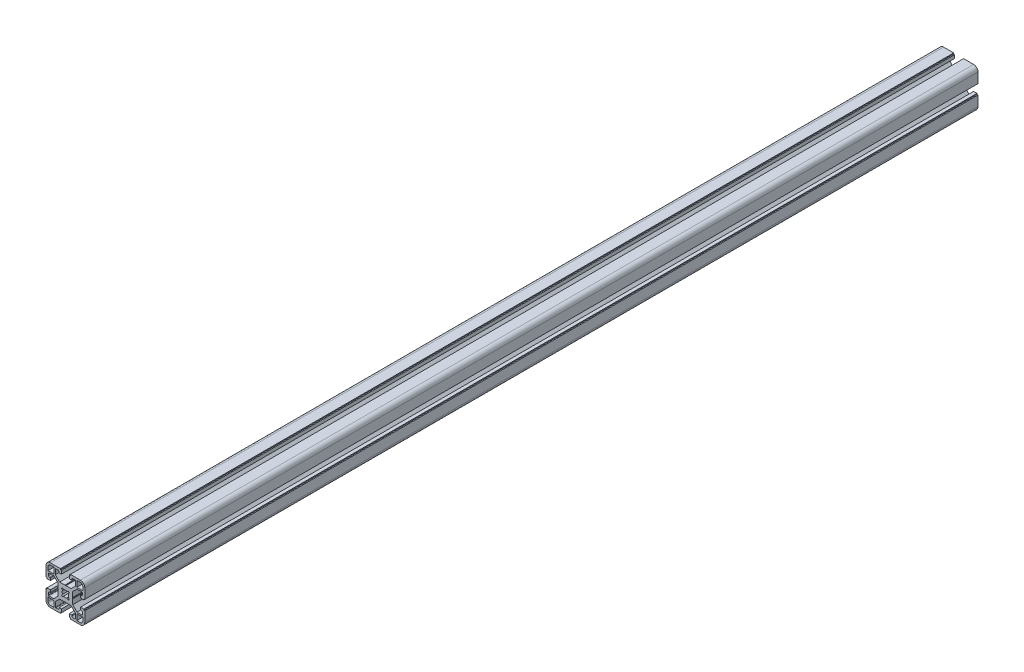
SolidWorks part; units mm, degrees
material "6061 GB/T6892-2006"
ref_plane "前视" through (0, 0, 0) normal (0, 0, 1) x (1, 0, 0)
ref_plane "上视" through (0, 0, 0) normal (0, 1, 0) x (1, 0, 0)
ref_plane "右视" through (0, 0, 0) normal (1, 0, 0) x (0, 0, -1)
sketch "草图1" plane through (0, 0, 0) normal (0, 0, 1) x (1, 0, 0)
  line L0 (-18.9995, -4.1003) -> (-18.9995, -5.1003)
  line L1 (-18.9995, -5.1003) -> (-19.9995, -5.1003)
  line L2 (-19.9995, -5.1003) -> (-19.9995, -15.5003)
  line L3 (-15.4995, -20.0003) -> (-5.0995, -20.0003)
  line L4 (-5.0995, -20.0003) -> (-5.0995, -19.0003)
  line L5 (-5.0995, -19.0003) -> (-4.0995, -19.0003)
  line L6 (-4.0995, -19.0003) -> (-4.0995, -15.5003)
  line L7 (-4.0995, -15.5003) -> (-6.5995, -15.5003)
  line L8 (-6.5995, -15.5003) -> (-6.5995, -16.5003)
  line L9 (-7.5995, -17.5003) -> (-9.7995, -17.5003)
  line L10 (-10.2995, -17.0003) -> (-10.2995, -11.9973)
  line L11 (-10.2995, -11.9973) -> (-5.9025, -7.6003)
  line L12 (-5.9025, -7.6003) -> (-0.5195, -7.6003)
  line L13 (-0.5195, -7.6003) -> (0.0005, -7.3003)
  line L14 (0.0005, -7.3003) -> (0.5195, -7.6003)
  line L15 (0.5195, -7.6003) -> (5.9035, -7.6003)
  line L16 (5.9035, -7.6003) -> (10.3005, -11.9973)
  line L17 (10.3005, -11.9973) -> (10.3005, -17.0003)
  line L18 (9.8005, -17.5003) -> (7.6005, -17.5003)
  line L19 (6.6005, -16.5003) -> (6.6005, -15.5003)
  line L20 (6.6005, -15.5003) -> (4.1005, -15.5003)
  line L21 (4.1005, -15.5003) -> (4.1005, -19.0003)
  line L22 (4.1005, -19.0003) -> (5.1005, -19.0003)
  line L23 (5.1005, -19.0003) -> (5.1005, -20.0003)
  line L24 (5.1005, -20.0003) -> (15.5005, -20.0003)
  line L25 (20.0005, -15.5003) -> (20.0005, -5.1003)
  line L26 (20.0005, -5.1003) -> (19.0005, -5.1003)
  line L27 (19.0005, -5.1003) -> (19.0005, -4.1003)
  line L28 (19.0005, -4.1003) -> (15.5005, -4.1003)
  line L29 (15.5005, -4.1003) -> (15.5005, -6.6003)
  line L30 (15.5005, -6.6003) -> (16.5005, -6.6003)
  line L31 (17.5005, -7.6003) -> (17.5005, -9.8003)
  line L32 (17.0005, -10.3003) -> (11.9975, -10.3003)
  line L33 (11.9975, -10.3003) -> (7.6005, -5.9033)
  line L34 (7.6005, -5.9033) -> (7.6005, -0.5203)
  line L35 (7.6005, -0.5203) -> (7.3005, -0.0003)
  line L36 (7.3005, -0.0003) -> (7.6005, 0.5197)
  line L37 (7.6005, 0.5197) -> (7.6005, 5.9027)
  line L38 (7.6005, 5.9027) -> (11.9975, 10.2997)
  line L39 (11.9975, 10.2997) -> (17.0005, 10.2997)
  line L40 (17.5005, 9.7997) -> (17.5005, 7.5997)
  line L41 (16.5005, 6.5997) -> (15.5005, 6.5997)
  line L42 (15.5005, 6.5997) -> (15.5005, 4.0997)
  line L43 (15.5005, 4.0997) -> (19.0005, 4.0997)
  line L44 (19.0005, 4.0997) -> (19.0005, 5.0997)
  line L45 (19.0005, 5.0997) -> (20.0005, 5.0997)
  line L46 (20.0005, 5.0997) -> (20.0005, 15.4997)
  line L47 (15.5005, 19.9997) -> (5.1005, 19.9997)
  line L48 (5.1005, 19.9997) -> (5.1005, 18.9997)
  line L49 (5.1005, 18.9997) -> (4.1005, 18.9997)
  line L50 (4.1005, 18.9997) -> (4.1005, 15.4997)
  line L51 (4.1005, 15.4997) -> (6.6005, 15.4997)
  line L52 (7.6005, 17.4997) -> (9.8005, 17.4997)
  line L53 (10.3005, 16.9997) -> (10.3005, 11.9967)
  line L54 (10.3005, 11.9967) -> (5.9035, 7.5997)
  line L55 (5.9035, 7.5997) -> (0.5195, 7.5997)
  line L56 (0.5195, 7.5997) -> (0.0005, 7.2997)
  line L57 (0.0005, 7.2997) -> (-0.5195, 7.5997)
  line L58 (-0.5195, 7.5997) -> (-5.9025, 7.5997)
  line L59 (-5.9025, 7.5997) -> (-10.2995, 11.9967)
  line L60 (-10.2995, 11.9967) -> (-10.2995, 16.9997)
  line L61 (-9.7995, 17.4997) -> (-7.5995, 17.4997)
  line L62 (-6.5995, 16.4997) -> (-6.5995, 15.4997)
  line L63 (-6.5995, 15.4997) -> (-4.0995, 15.4997)
  line L64 (-4.0995, 15.4997) -> (-4.0995, 18.9997)
  line L65 (-4.0995, 18.9997) -> (-5.0995, 18.9997)
  line L66 (-5.0995, 18.9997) -> (-5.0995, 19.9997)
  line L67 (-5.0995, 19.9997) -> (-15.4995, 19.9997)
  line L68 (-19.9995, 15.4997) -> (-19.9995, 5.0997)
  line L69 (-19.9995, 5.0997) -> (-18.9995, 5.0997)
  line L70 (-18.9995, 5.0997) -> (-18.9995, 4.0997)
  line L71 (-18.9995, 4.0997) -> (-15.4995, 4.0997)
  line L72 (-15.4995, 4.0997) -> (-15.4995, 6.5997)
  line L73 (-15.4995, 6.5997) -> (-16.4995, 6.5997)
  line L74 (-17.4995, 7.5997) -> (-17.4995, 9.7997)
  line L75 (-16.9995, 10.2997) -> (-11.9965, 10.2997)
  line L76 (-11.9965, 10.2997) -> (-7.5995, 5.9027)
  line L77 (-7.5995, 5.9027) -> (-7.5995, 0.5197)
  line L78 (-7.5995, 0.5197) -> (-7.2995, -0.0003)
  line L79 (-7.2995, -0.0003) -> (-7.5995, -0.5203)
  line L80 (-7.5995, -0.5203) -> (-7.5995, -5.9033)
  line L81 (-7.5995, -5.9033) -> (-11.9965, -10.3003)
  line L82 (-11.9965, -10.3003) -> (-16.9995, -10.3003)
  line L83 (-17.4995, -9.8003) -> (-17.4995, -7.6003)
  line L84 (-16.4995, -6.6003) -> (-15.4995, -6.6003)
  line L85 (-15.4995, -6.6003) -> (-15.4995, -4.1003)
  line L86 (-15.4995, -4.1003) -> (-18.9995, -4.1003)
  line L87 (15.5005, -18.0003) -> (11.8005, -18.0003)
  line L88 (11.8005, -18.0003) -> (11.8005, -11.8003)
  line L89 (11.8005, -11.8003) -> (18.0005, -11.8003)
  line L90 (18.0005, -11.8003) -> (18.0005, -15.5003)
  line L91 (18.0005, 11.7997) -> (11.8005, 11.7997)
  line L92 (11.8005, 11.7997) -> (11.8005, 17.9997)
  line L93 (11.8005, 17.9997) -> (15.5005, 17.9997)
  line L94 (18.0005, 15.4997) -> (18.0005, 11.7997)
  line L95 (-1.8145, -2.8753) -> (-3.0044, -4.0665)
  line L96 (-3.0044, -4.0665) -> (-4.0656, -3.0052)
  line L97 (-4.0656, -3.0052) -> (-2.8745, -1.8153)
  line L98 (-2.8745, 1.8147) -> (-4.0644, 3.0058)
  line L99 (-4.0644, 3.0058) -> (-3.0044, 4.0658)
  line L100 (-3.0044, 4.0658) -> (-1.8145, 2.8747)
  line L101 (1.8145, 2.8747) -> (3.0055, 4.0657)
  line L102 (3.0055, 4.0657) -> (4.0666, 3.0045)
  line L103 (4.0666, 3.0045) -> (2.8755, 1.8147)
  line L104 (2.8755, -1.8153) -> (4.0666, -3.0052)
  line L105 (4.0666, -3.0052) -> (3.0055, -4.0663)
  line L106 (3.0055, -4.0663) -> (1.8145, -2.8753)
  line L107 (-17.9995, -15.5003) -> (-17.9995, -11.8003)
  line L108 (-17.9995, -11.8003) -> (-11.7995, -11.8003)
  line L109 (-11.7995, -11.8003) -> (-11.7995, -18.0003)
  line L110 (-11.7995, -18.0003) -> (-15.4995, -18.0003)
  line L111 (-11.7995, 17.9997) -> (-11.7995, 11.7997)
  line L112 (-11.7995, 11.7997) -> (-17.9995, 11.7997)
  line L113 (-17.9995, 11.7997) -> (-17.9995, 15.4997)
  line L114 (-15.4995, 17.9997) -> (-11.7995, 17.9997)
  arc A0 (-19.9995, -15.5003) -> (-15.4995, -20.0003) centre (-15.4995, -15.5003) ccw
  arc A1 (-6.5995, -16.5003) -> (-7.5995, -17.5003) centre (-7.5995, -16.5003) cw
  arc A2 (-9.7995, -17.5003) -> (-10.2995, -17.0003) centre (-9.7995, -17.0003) cw
  arc A3 (10.3005, -17.0003) -> (9.8005, -17.5003) centre (9.8005, -17.0003) cw
  arc A4 (7.6005, -17.5003) -> (6.6005, -16.5003) centre (7.6005, -16.5003) cw
  arc A5 (15.5005, -20.0003) -> (20.0005, -15.5003) centre (15.5005, -15.5003) ccw
  arc A6 (16.5005, -6.6003) -> (17.5005, -7.6003) centre (16.5005, -7.6003) cw
  arc A7 (17.5005, -9.8003) -> (17.0005, -10.3003) centre (17.0005, -9.8003) cw
  arc A8 (17.0005, 10.2997) -> (17.5005, 9.7997) centre (17.0005, 9.7997) cw
  arc A9 (17.5005, 7.5997) -> (16.5005, 6.5997) centre (16.5005, 7.5997) cw
  arc A10 (20.0005, 15.4997) -> (15.5005, 19.9997) centre (15.5005, 15.4997) ccw
  arc A11 (6.6005, 15.4997) -> (6.6005, 16.4997) centre (7.1003, 15.9997) cw
  arc A12 (6.6005, 16.4997) -> (7.6005, 17.4997) centre (7.6005, 16.4997) cw
  arc A13 (9.8005, 17.4997) -> (10.3005, 16.9997) centre (9.8005, 16.9997) cw
  arc A14 (-10.2995, 16.9997) -> (-9.7995, 17.4997) centre (-9.7995, 16.9997) cw
  arc A15 (-7.5995, 17.4997) -> (-6.5995, 16.4997) centre (-7.5995, 16.4997) cw
  arc A16 (-15.4995, 19.9997) -> (-19.9995, 15.4997) centre (-15.4995, 15.4997) ccw
  arc A17 (-16.4995, 6.5997) -> (-17.4995, 7.5997) centre (-16.4995, 7.5997) cw
  arc A18 (-17.4995, 9.7997) -> (-16.9995, 10.2997) centre (-16.9995, 9.7997) cw
  arc A19 (-16.9995, -10.3003) -> (-17.4995, -9.8003) centre (-16.9995, -9.8003) cw
  arc A20 (-17.4995, -7.6003) -> (-16.4995, -6.6003) centre (-16.4995, -7.6003) cw
  arc A21 (18.0005, -15.5003) -> (15.5005, -18.0003) centre (15.5005, -15.5003) cw
  arc A22 (15.5005, 17.9997) -> (18.0005, 15.4997) centre (15.5005, 15.4997) cw
  arc A23 (-2.8745, -1.8153) -> (-2.8745, 1.8147) centre (0.0005, -0.0003) cw
  arc A24 (-1.8145, 2.8747) -> (1.8145, 2.8747) centre (0, -0.0007) cw
  arc A25 (2.8755, 1.8147) -> (2.8755, -1.8153) centre (0.0005, -0.0003) cw
  arc A26 (1.8145, -2.8753) -> (-1.8145, -2.8753) centre (0, 0) cw
  arc A27 (-15.4995, -18.0003) -> (-17.9995, -15.5003) centre (-15.4995, -15.5003) cw
  arc A28 (-17.9995, 15.4997) -> (-15.4995, 17.9997) centre (-15.4995, 15.4997) cw
extrude "凸台-拉伸1" add sketch "草图1" against normal blind 922
